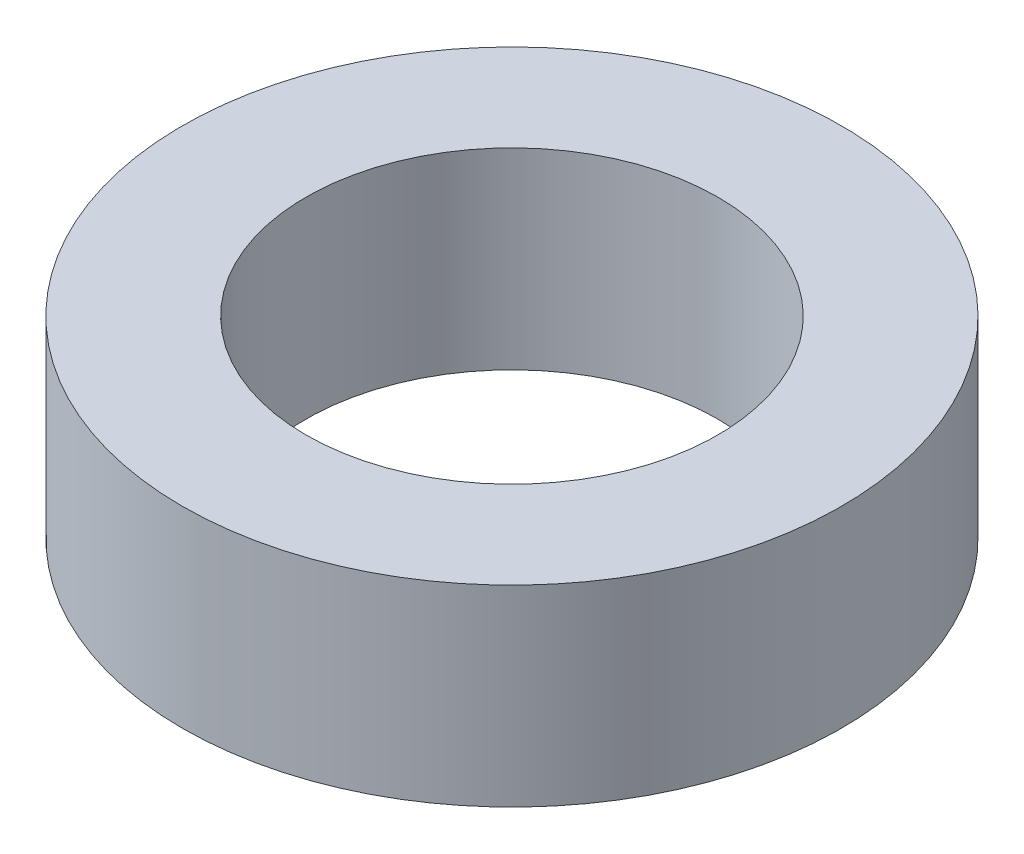
from build123d import *

# Parameters (mm, degrees)
SKETCH2_R           = 12
SKETCH2_R_2         = 7.5
BOSS_EXTRUDE1_DEPTH = 7


with BuildPart() as part:
    # Sketch2 → Boss-Extrude1 (new body)
    with BuildSketch(Plane(origin=(0, 0, 0), x_dir=(1, 0, 0), z_dir=(0, 1, 0))):
        with Locations(Location((0, 0, 0), (0, 0, 270))):
            Circle(SKETCH2_R)
        with Locations(Location((0, 0, 0), (0, 0, 270))):
            Circle(SKETCH2_R_2, mode=Mode.SUBTRACT)
    extrude(amount=BOSS_EXTRUDE1_DEPTH)


solid = part.part
